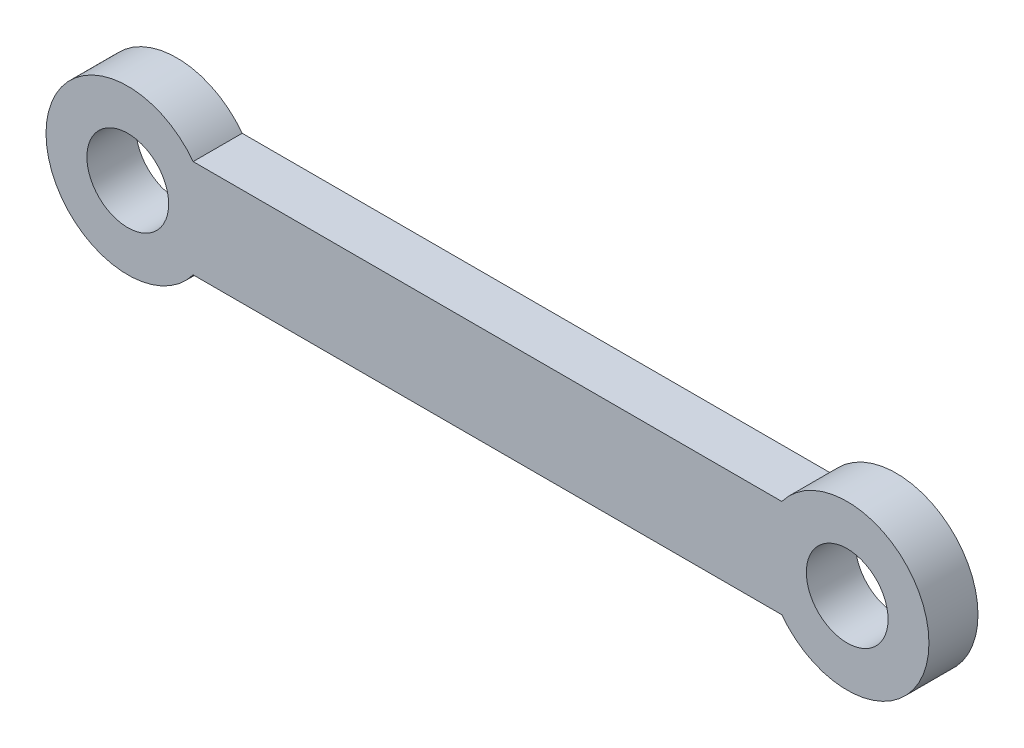
SolidWorks part; units mm, degrees
ref_plane "Front Plane" through (0, 0, 0) normal (0, 0, 1) x (1, 0, 0)
ref_plane "Top Plane" through (0, 0, 0) normal (0, 1, 0) x (1, 0, 0)
ref_plane "Right Plane" through (0, 0, 0) normal (1, 0, 0) x (0, 0, -1)
sketch "Sketch1" plane through (0, 0, 0) normal (0, 0, 1) x (1, 0, 0)
  line L2 (0, 0) -> (44, 0) construction
  line L3 (4, 3) -> (40, 3)
  line L4 (4, -3) -> (40, -3)
  circle A0 centre (0, 0) radius 2.5
  arc A1 (4, 3) -> (4, -3) centre (0, 0) ccw
  circle A2 centre (44, 0) radius 2.5
  arc A3 (40, -3) -> (40, 3) centre (44, 0) ccw
  dimension "D1" = 44
  dimension "D2" = 5
  dimension "D3" = 5
  dimension "D4" = 10
  dimension "D5" = 10
  dimension "D8" = 6
  dimension "D9" = 3
extrude "Boss-Extrude1" add sketch "Sketch1" along normal blind 3
